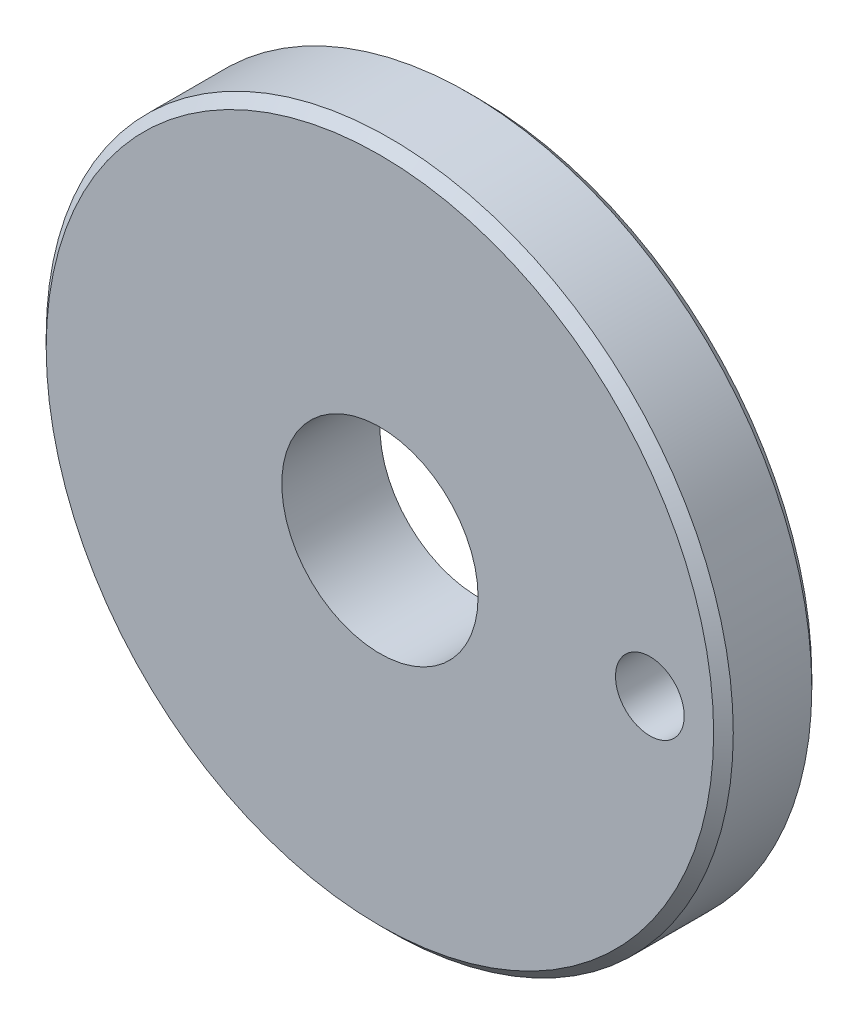
SolidWorks part; units mm, degrees
ref_plane "Front Plane" through (0, 0, 0) normal (0, 0, 1) x (1, 0, 0)
ref_plane "Top Plane" through (0, 0, 0) normal (0, 1, 0) x (1, 0, 0)
ref_plane "Right Plane" through (0, 0, 0) normal (1, 0, 0) x (0, 0, -1)
sketch "Sketch1" plane through (0, 0, 0) normal (0, 0, 1) x (1, 0, 0)
  circle A0 centre (0, 0) radius 35
  dimension "D1" = 70
extrude "Boss-Extrude1" add sketch "Sketch1" along normal blind 10
chamfer "Chamfer1" distance 1 angle 45 2 edges at (35, 0, 0) (35, 0, 10)
sketch "Sketch2" plane through (0, 0, 10) normal (0, 0, 1) x (1, 0, 0)
  circle A0 centre (0, 0) radius 10
  dimension "D1" = 20
extrude "Cut-Extrude1" cut sketch "Sketch2" against normal blind 30
sketch "Sketch3" plane through (0, 0, 10) normal (0, 0, 1) x (1, 0, 0)
  circle A1 centre (27.5, 0) radius 3.5
  dimension "D2" = 7
extrude "Cut-Extrude2" cut sketch "Sketch3" against normal blind 29
